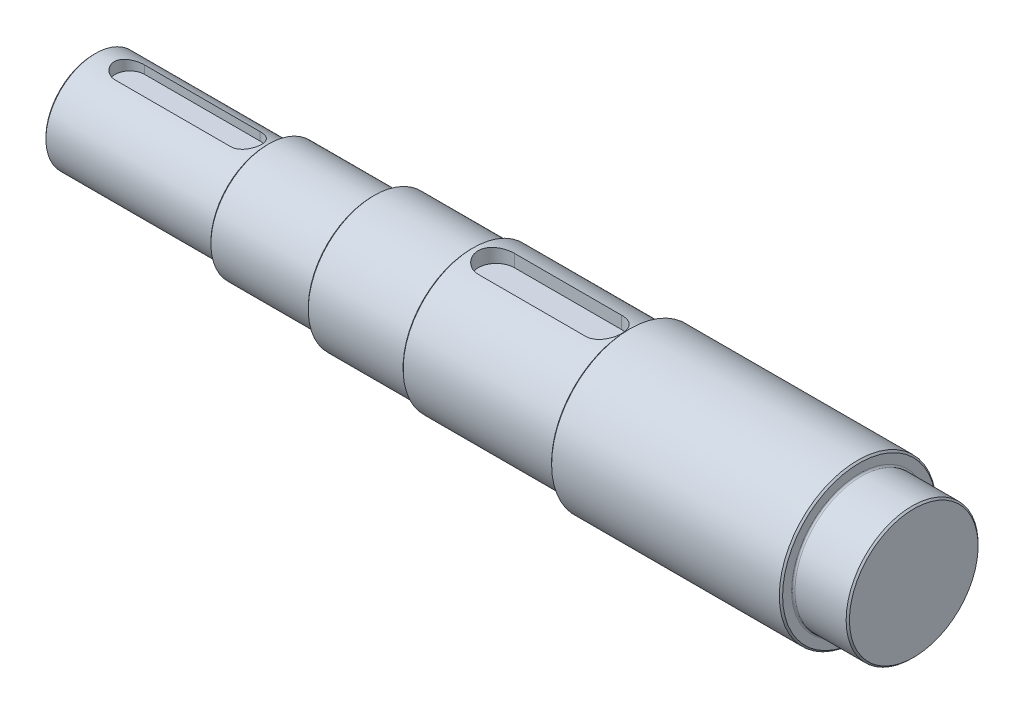
from build123d import *

# Parameters (mm, degrees)
CUT_EXTRUDE2_DEPTH = 9
CUT_EXTRUDE3_DEPTH = 7
CHAMFER1_SIZE      = 1
FILLET1_R          = 1


with BuildPart() as part:
    # Sketch1 → Revolve2 (revolve)
    with BuildSketch(Plane.XY, mode=Mode.PRIVATE) as revolve2_sk:
        Polygon((0, 0), (0, 30), (105, 30), (105, 35), (169, 35), (169, 40), (229, 40), (229, 42.5), (324, 42.5), (324, 47.5), (464, 47.5), (464, 40), (497, 40), (497, 0), align=None)
    revolve(revolve2_sk.sketch.rotate(Axis((-10.323535414, 0, 0), (1, 0, 0)), 90), axis=Axis((-10.323535414, 0, 0), (1, 0, 0)))

    # Sketch2 → Cut-Extrude2 (cut)
    with BuildSketch(Plane(origin=(0, 42.5, 0), x_dir=(1, 0, 0), z_dir=(0, 1, 0))):
        with BuildLine():
            Line((309, 11), (244, 11))
            ThreePointArc((244, 11), (233, 0), (244, -11))
            Line((244, -11), (309, -11))
            ThreePointArc((309, -11), (320, 0), (309, 11))
        make_face()
    extrude(amount=-CUT_EXTRUDE2_DEPTH, mode=Mode.SUBTRACT)

    # Sketch4 → Cut-Extrude3 (cut)
    with BuildSketch(Plane(origin=(0, 30, 0), x_dir=(1, 0, 0), z_dir=(0, 1, 0))):
        with BuildLine():
            Line((90, 10.905409347), (20, 10.905409347))
            ThreePointArc((20, 10.905409347), (11, 1.905409347), (20, -7.094590653))
            Line((20, -7.094590653), (90, -7.094590653))
            ThreePointArc((90, -7.094590653), (99, 1.905409347), (90, 10.905409347))
        make_face()
    extrude(amount=-CUT_EXTRUDE3_DEPTH, mode=Mode.SUBTRACT)

    # Chamfer1
    chamfer1_edges = [part.edges().sort_by_distance(p)[0] for p in [
        (497, 0, -40),
        (464, 0, -47.5),
        (324, 0, -47.5),
        (229, 0, -42.5),
        (169, 0, -40),
        (105, 0, -35),
        (0, 0, -30),
    ]]
    chamfer(chamfer1_edges, length=CHAMFER1_SIZE)

    # Fillet1
    fillet1_edges = [part.edges().sort_by_distance(p)[0] for p in [
        (464, 0, -40),
        (324, 0, -42.5),
        (229, 0, -40),
        (169, 0, -35),
        (105, 0, -30),
    ]]
    fillet(fillet1_edges, radius=FILLET1_R)


solid = part.part
